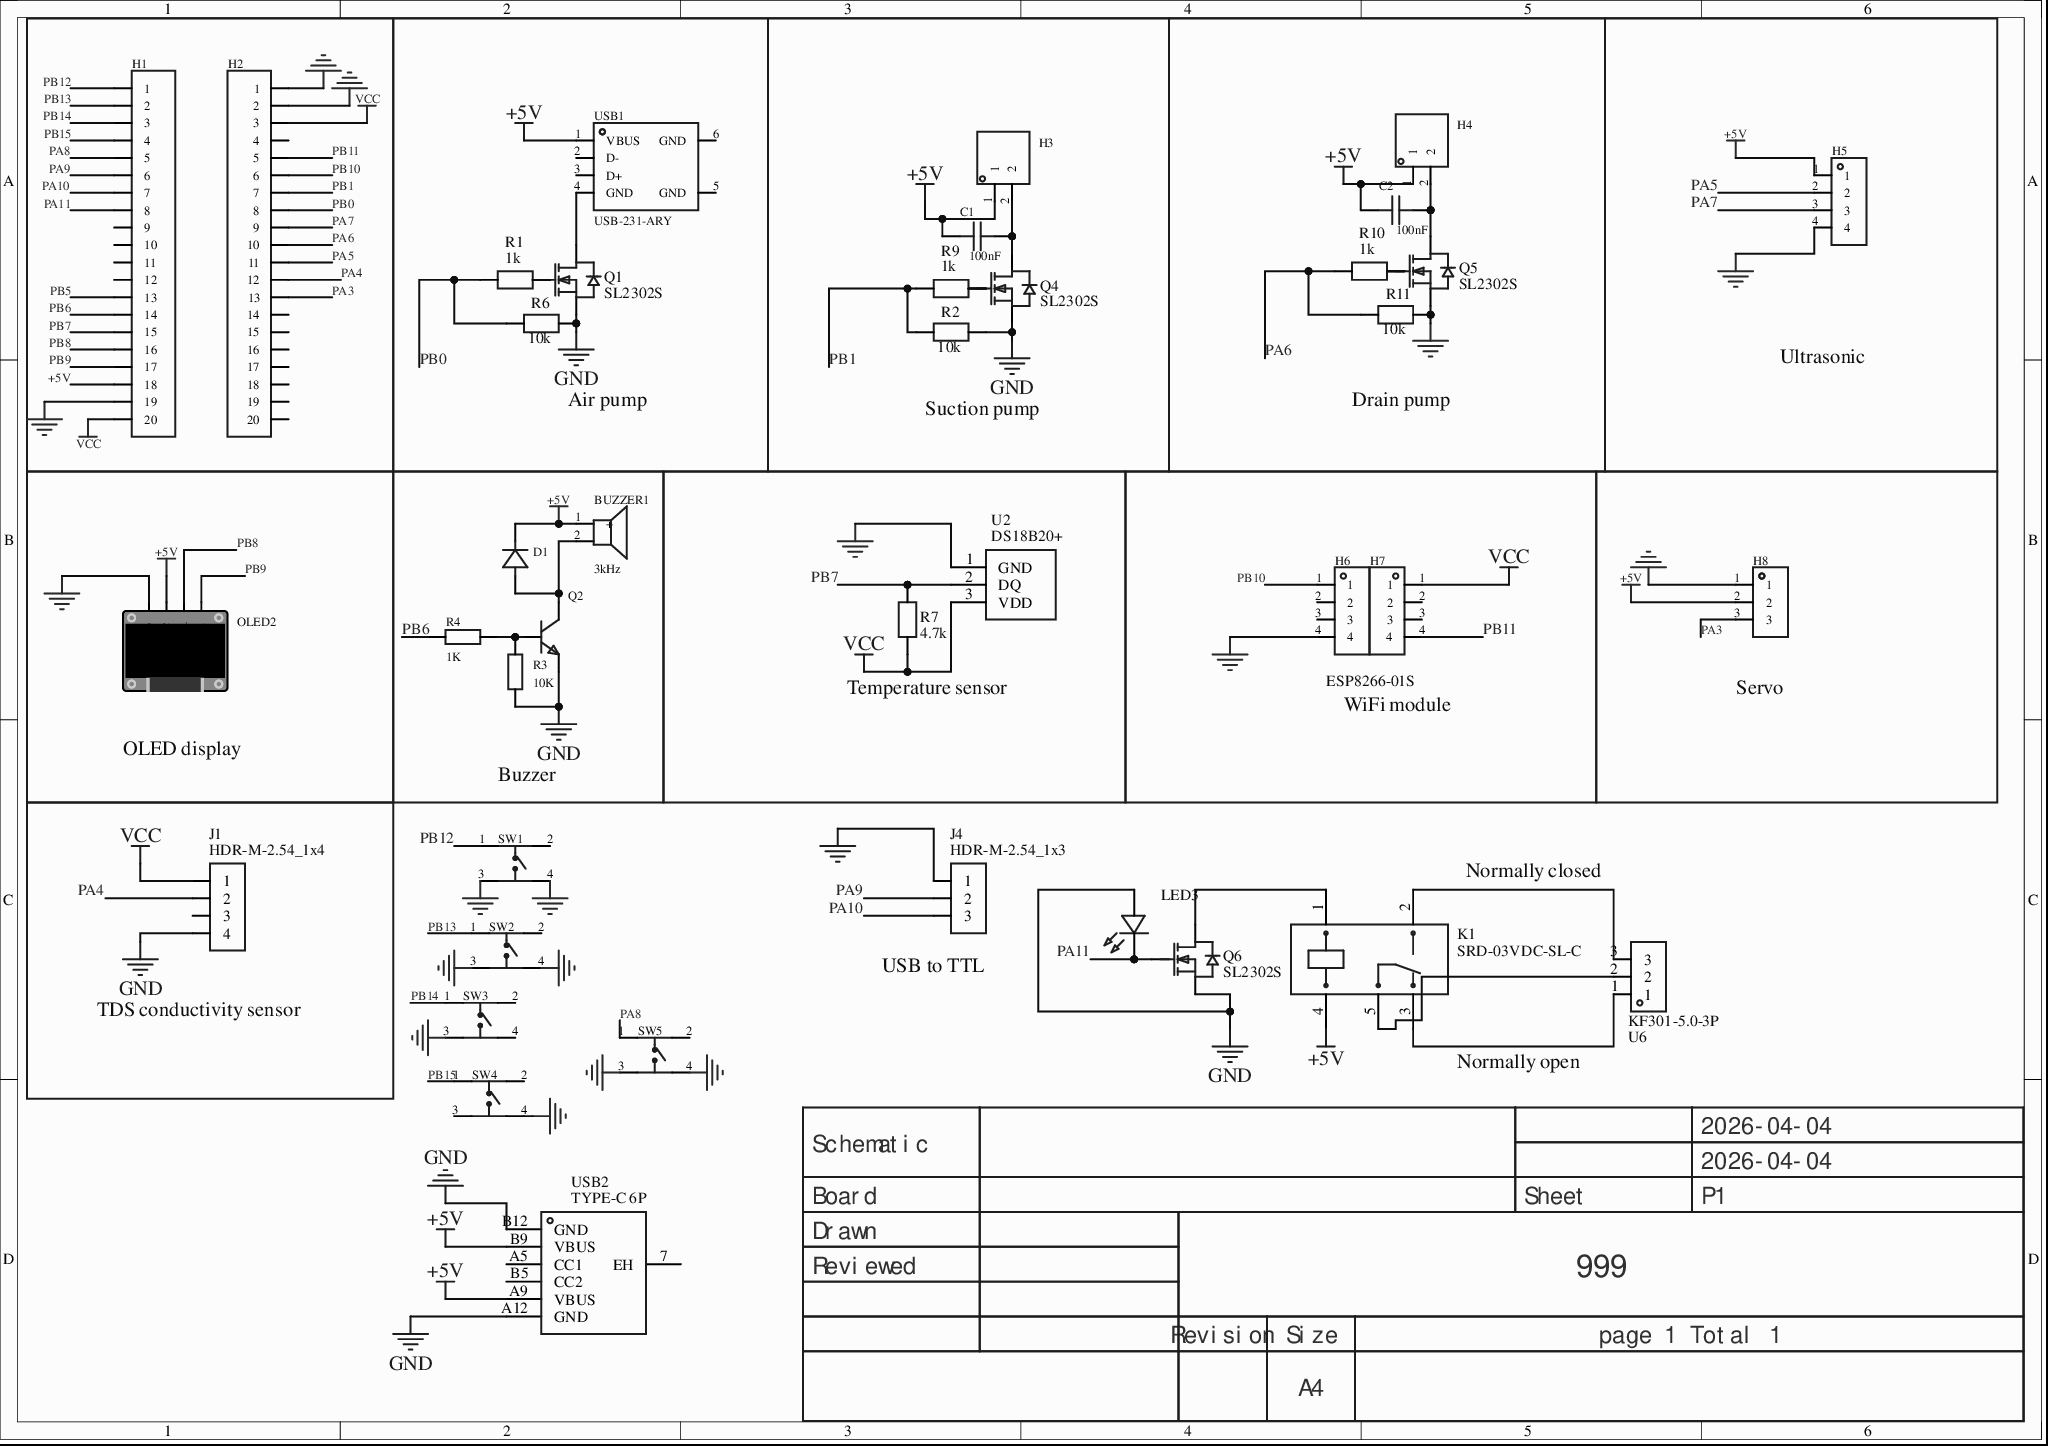
[diagram p0: MISC75353-3.schdoc]
# Altium project MISC75353-2.PrjPcb
1 sheet, 40 parts. Net scope: global (net labels, ports and power ports of the same name join across sheets).
Board file: MISC75353.pcbdoc

## Sheet MISC75353-3.schdoc
size 297 x 209 mm; Version: V1.0; @Project Name: MISC75353; @Update Date: 2026-04-04; @Create Date: 2026-04-04; @Board Name: MISC75353; @Create Time: 13:37:19; @Page Count: 1; @Page No: 1; @Schematic Name: MISC75353; @Update Time: 13:37:19; Size: A4

### Parts
BUZZER1  3kHz  [BUZ-TH_BD9.6-P5.00-D0.7-FD]
C1  100nF  [C0805]
C2  100nF  [C0805]
D1  (no value)  [DO_1N4007]
H1  (no value)  [HDR-TH_20P-P2.54-V-F]
H2  (no value)  [HDR-TH_20P-P2.54-V-F]
H3  (no value)  [HDR-TH_2P-P2.54-V-M-1]
H4  (no value)  [HDR-TH_2P-P2.54-V-M-1]
H5  (no value)  [HDR-TH_4P-P2.54-V-M]
H6  (no value)  [HDR-TH_4P-P2.54-V-M]
H7  (no value)  [HDR-TH_4P-P2.54-V-M]
H8  (no value)  [HDR-TH_3P-P2.54-V-M]
J1  HDR-M-2.54_1x4  [HDR-M-2.54_1X4]
J4  HDR-M-2.54_1x3  [HDR-M-2.54_1X3]
K1  SRD-03VDC-SL-C  [RELAY-TH_SRD-XXVDC-XL-C]
LED3  LED-TH-5mm_R  [LED-TH_BD5.0_RED]  (value not drawn)
OLED2  (no value)  [0.96OLED_4P]
Q1  SL2302S  [SOT-23_L2.9-W1.3-P1.90-LS2.4-BR]
Q2  (no value)  [S8050_TO_92]
Q4  SL2302S  [SOT-23_L2.9-W1.3-P1.90-LS2.4-BR]
Q5  SL2302S  [SOT-23_L2.9-W1.3-P1.90-LS2.4-BR]
Q6  SL2302S  [SOT-23_L2.9-W1.3-P1.90-LS2.4-BR]
R1  1k  [R0603]
R2  10k  [R0603]
R3  10K  [R0603]
R4  1K  [R0603]
R6  10k  [R0603]
R7  4.7k  [R0603]
R9  1k  [R0603]
R10  1k  [R0603]
R11  10k  [R0603]
SW1  J1L0503110  [SW-TH_4P-L6.0-W6.0-P4.50-LS6.3]  (value not drawn)
SW2  J1L0503110  [SW-TH_4P-L6.0-W6.0-P4.50-LS6.3]  (value not drawn)
SW3  J1L0503110  [SW-TH_4P-L6.0-W6.0-P4.50-LS6.3]  (value not drawn)
SW4  J1L0503110  [SW-TH_4P-L6.0-W6.0-P4.50-LS6.3]  (value not drawn)
SW5  J1L0503110  [SW-TH_4P-L6.0-W6.0-P4.50-LS6.3]  (value not drawn)
U2  DS18B20+  [TO-92-3_L4.9-W3.7-P1.27-L]
U6  KF301-5.0-3P  [CONN-TH_3P-P5.00_KF301-5.0-3P]
USB1  USB-231-ARY  [USB-A-TH_USB-231-ARY]
USB2  TYPE-C 6P  [TYPE-C-SMD_TYPE-C-6P_1]

### Blocks framed on the sheet
Air pump: Q1 R1 R6 USB1
Suction pump: C1 H3 Q4 R2 R9
Drain pump: C2 H4 Q5 R10 R11
Ultrasonic: H5
OLED display: OLED2
Buzzer: BUZZER1 D1 Q2 R3 R4
Temperature sensor: R7 U2
WiFi module: H6 H7
Servo: H8
TDS conductivity sensor: J1

### Nets
+5V: BUZZER1.1(+) C1.1 C2.1 D1.1(K) H1.18 H3.1 H4.1 H5.1 H8.2 K1.4 OLED2.2(VCC) USB1.1(VBUS) USB2.A9(VBUS) USB2.B9(VBUS)
GND: H1.19 H2.1 H2.2 H5.4 H6.4 H8.1 J1.4 J4.1 LED3.1 OLED2.1(GND) Q1.2(S) Q2.1(E) Q4.2(S) Q5.2(S) Q6.2(S) R2.2 R3.1 R6.2 R11.2 SW1.3 SW1.4 SW2.3 SW2.4 SW3.3 SW4.4 SW5.3 SW5.4 U2.1(GND) USB2.A12(GND) USB2.B12(GND)
VCC: H1.20 H2.3 H7.1 J1.1 R7.2 U2.3(VDD)
PA3: H2.13 H8.3
PA4: H2.12 J1.2
PA5: H2.11 H5.2
PA6: H2.10 R10.1 R11.1
PA7: H2.9 H5.3
PA8: H1.5 SW5.1
PA9: H1.6 J4.2
PA10: H1.7 J4.3
PA11: H1.8 LED3.2 Q6.1(G)
PB0: H2.8 R1.1 R6.1
PB1: H2.7 R2.1 R9.1
PB5: H1.13
PB6: H1.14 R4.2
PB7: H1.15 R7.1 U2.2(DQ)
PB8: H1.16 OLED2.3(SCL)
PB9: H1.17 OLED2.4(SDA)
PB10: H2.6 H6.1
PB11: H2.5 H7.4
PB12: H1.1 SW1.1
PB13: H1.2 SW2.1
PB14: H1.3 SW3.1
PB15: H1.4 SW4.1
NetBUZZER1_2: BUZZER1.2 D1.2(A) Q2.3(C)
NetC1_2: C1.2 H3.2 Q4.3(D)
NetC2_2: C2.2 H4.2 Q5.3(D)
NetK1_1: K1.1 Q6.3(D)
NetK1_2: K1.2 U6.3
NetK1_3: K1.3 U6.1
NetK1_5: K1.5 U6.2
NetQ1_1: Q1.1(G) R1.2
NetQ1_3: Q1.3(D) USB1.4(GND)
NetQ2_2: Q2.2(B) R3.2 R4.1
NetQ4_1: Q4.1(G) R9.2
NetQ5_1: Q5.1(G) R10.2

Not connected (* = marked no-connect by the designer): H1 9 10 11 12; H2 4 14 15 16 17 18 19 20; H6 2* 3*; H7 2* 3*; J1 3*; SW1 2*; SW2 2*; SW3 2* 4*; SW4 2* 3*; SW5 2*; USB1 2(D-)* 3(D+)* 5(GND)* 6(GND)*; USB2 7(EH)* A5(CC1)* B5(CC2)*

### Notes on the sheet
- ESP8266-01S
- Normally closed
- (near J4) USB to TTL
- Normally open
- 2026-04-04
- Schematic
- Board
- Sheet
- P1
- Drawn
- Reviewed
- 999
- Revision
- Size
- A4
- page 1 Total 1

### Library data of the parts
BUZZER1 = HNB09A05: Driver type: active (built-in driver circuit); construction type: electromagnetic; rated voltage: -; frequency: 3kHz; sound pressure (SPL): 85dB;; Manufacturer: 华能; 3D Model: 13273335caac486e928bafb4d9fdf12d0819f05c4eef4c71ace90d822a990e87; 3D Model Transform: 354.33,354.33,0,90,0,0,0,0,-177.165; Voltage - Supply: 3V~7V; AddInBom: yes; ModelName: BUZ-TH_D9.0-H5.5-P5.0; Symbol: HNB09A05; Device: HNB09A05; LCSC Part Name: HNB09A05; Supplier Part: C96493; Manufacturer Part: HNB09A05; Supplier Footprint: 插件,D=9mm; JLCPCB Part Class: Extended Part; Datasheet: https://example.com/datasheet/HNB09A05/97698.html; Supplier: LCSC; Driver Circuitry: Active (built-in driver circuit); Technology: Electromagnetic; Voltage Rating: -; Value: 3kHz; Current Consumption: -; Sound Pressure Level(SPL): 85dB; Diameter(φD): 9mm; Length: -; Width: -; Height: 5.7mm; Operating Temperature: -; ConvertToPcb: yes; FootprintName: BUZ-TH_BD9.6-P5.00-D0.7-FD
C1 C2 = CAP_0805: Symbol: Capacitance; ConvertToPcb: yes; ModelId: 1ba041120af144c991958decab20d2410819f05c4eef4c71ace90d822a990e87; ModelName: C0805_L2.0-W1.3-H1.3; ModelTransform: 78.74,51.181,0,0,0,0,0,0.0005,0; Device: CAP_0805; AddInBom: yes; Supplier Footprint: 0805; FootprintName: C0805; Value: 100nF
D1 = D_1N4007A: AddInBom: yes; ModelId: 6de1e9b71a0d4751b4e9df530304c1a30819f05c4eef4c71ace90d822a990e87; ModelName: DO-41_D2.4-L4.7-P8.70; ModelTransform: 373.9,94.4,232.29,0,0,0,0,0,-140; Symbol: D_1N4007; Device: D_1N4007A; Supplier Footprint: DO-41; ConvertToPcb: yes; FootprintName: DO_1N4007
H1 H2 = HDR-F_2.54_1x20P: 3D Model: db7015f7ad9d48b8a3b1188db02e34290819f05c4eef4c71ace90d822a990e87; 3D Model Transform: 1999.996,100,0,0,0,0,0,0,-118.11; ConvertToPcb: yes; ModelName: HDR-F-2.54_1x20; Symbol: HDR-F_2.54_1x20P; Device: HDR-F_2.54_1x20P; Supplier Part: C50984; Supplier Footprint: 插件; AddInBom: yes; FootprintName: HDR-TH_20P-P2.54-V-F
H3 H4 = HDR-M_2.54_1x2P: Symbol: 210S-1*2P L=11.6MMGold-plated black; ConvertToPcb: yes; ModelId: 79b2e9f2d70a4d68a1b7098f27c6d4c50819f05c4eef4c71ace90d822a990e87; ModelName: HDR-M-2.54_1x2; ModelTransform: 200,100,0,0,0,0,0,0,-118.11; Device: HDR-M_2.54_1x2P; AddInBom: yes; SupplierPart: C124375; Supplier Footprint: 插件; FootprintName: HDR-TH_2P-P2.54-V-M-1
H5-H7 = HDR-M_2.54_1x4P: Symbol: PZ254V-11-04P; ConvertToPcb: yes; ModelId: 112f4d05e8d64e99ab9a333894bea4f90819f05c4eef4c71ace90d822a990e87; ModelName: HDR-TH_4P-P2.54-M-LI-1X4P; ModelTransform: 399.999,104.7242,0,0,0,0,0,0,-118.11; Device: HDR-M_2.54_1x4P; AddInBom: yes; SupplierPart: C492403; Supplier Footprint: 插件; FootprintName: HDR-TH_4P-P2.54-V-M
H8 = HDR-M_2.54_1x3P: AddInBom: yes; ModelId: bb473b6d38ff42a99216a4fcdbdcc4cb0819f05c4eef4c71ace90d822a990e87; ModelName: HDR-TH_3P-P2.54-M-LI-1X3P; ModelTransform: 300.03877,100,0,0,0,0,0,0,-118.11; Symbol: HDR-M_2.54_1x3P; Device: HDR-M_2.54_1x3P; ConvertToPcb: yes; FootprintName: HDR-TH_3P-P2.54-V-M; SupplierPart: C2937625; Supplier Footprint: 插件
J1 = HDR-M-2.54_1x4: Add into BOM: yes; ModelId: cd502121c3eb48dbbf0ecbc8e7ad097f; Symbol: HDR-M-2.54_1x4; Device: HDR-M-2.54_1x4; Convert to PCB: yes; Supplier Part: C124378; Supplier: LCSC; Origin 3D Model Title: HDR-M-2.54_1X4; FootprintName: HDR-M-2.54_1X4; ModelName: HDR-M-2.54_1X4
J4 = HDR-M-2.54_1x3: Add into BOM: yes; ModelId: e45037aab22c4927a5ea885f2a5b96c9; Symbol: HDR-M-2.54_1x3; Device: HDR-M-2.54_1x3; Convert to PCB: yes; Supplier Part: C180248; Supplier: LCSC; Origin 3D Model Title: HDR-M-2.54_1x3; FootprintName: HDR-M-2.54_1X3; ModelName: HDR-M-2.54_1x3
K1 = SRD-03VDC-SL-C: Manufacturer: 松乐; Add into BOM: yes; Origin 3D Model Title: RELAY-TH_L19.2-W15.6-H15.8; ModelId: d0eda9b8bf8746d18ae810ab88dc78e7; Symbol: SRD-03VDC-SL-C; Device: SRD-03VDC-SL-C; Convert to PCB: yes; Supplier: LCSC; Manufacturer Part: SRD-03VDC-SL-C; Supplier Part: C24585; JLCPCB Part Class: Extended Part; FootprintName: RELAY-TH_SRD-XXVDC-XL-C; ModelName: RELAY-TH_L19.2-W15.6-H15.8
LED3 = LED-TH-5mm_R: Manufacturer: EVERLIGHT(台湾亿光); Manufacturer Part: 333-2SURD/S530-A3; Add into BOM: yes; ModelId: 0e3e1c3f5c0d4d279dc0d0ab1929e6bc; Symbol: LED-TH-5mm_R; Device: LED-TH-5mm_R; Convert to PCB: yes; Supplier Part: C87271; Supplier: LCSC; Origin 3D Model Title: LED-TH_BD5.0_Red; FootprintName: LED-TH_BD5.0_RED; ModelName: LED-TH_BD5.0_Red
OLED2 = 0.96OLED模块_4P: Symbol: 0.96OLED module_4P; ConvertToPcb: yes; ModelId: 79c000fdb68d45a296c2e9bedf4f90550819f05c4eef4c71ace90d822a990e87; ModelTransform: 1393.69792,1318.895,0,0,0,0,0,-560.079,-137.795; Device: 0.96OLED module_4P; AddInBom: yes; FootprintName: 0.96OLED_4P; Supplier Footprint: 插件; ModelName: 0.96OLED_4P
Q1 Q4-Q6 = SL2302S: Manufacturer: Slkor(萨科微); Add into BOM: yes; Origin 3D Model Title: SOT-23-3P_L2.9-W1.3-H1.0-LS2.4-P0.95; ModelId: c62791f0466c4ae2a892c056b845b0ca; Symbol: SL2302S; Device: SL2302S; Convert to PCB: yes; Supplier: LCSC; Supplier Part: C473811; Manufacturer Part: SL2302S; JLCPCB Part Class: Extended Part; FootprintName: SOT-23_L2.9-W1.3-P1.90-LS2.4-BR; ModelName: SOT-23-3P_L2.9-W1.3-H1.0-LS2.4-P0.95
Q2 = S8050_TO_NPN: ConvertToPcb: yes; ModelId: aafe8e06f2154e7c93506efd0d6632dd0819f05c4eef4c71ace90d822a990e87; ModelName: TO-92-3_L4.9-W3.7-P1.27-L; ModelTransform: 180.78,141.44,417.3,0,0,0,0,0,-200; Symbol: S8050_TO_NPN; Device: S8050_TO_NPN; AddInBom: yes; Supplier Footprint: TO-92; FootprintName: S8050_TO_92
R1 R9 R10 = 1k: Add into BOM: yes; ModelId: fc143cca1e79419f9cd78b61e9279f08; Symbol: 1k; Device: 1k; Convert to PCB: yes; Origin 3D Model Title: R0603; FootprintName: R0603; ModelName: R0603
R2 R6 R7 R11 = 10k: Add into BOM: yes; ModelId: fc143cca1e79419f9cd78b61e9279f08; Symbol: 10k; Device: 10k; Convert to PCB: yes; Origin 3D Model Title: R0603; FootprintName: R0603; ModelName: R0603
R3 R4 = Res_0603: Symbol: Resistor; ConvertToPcb: yes; ModelId: fc143cca1e79419f9cd78b61e9279f080819f05c4eef4c71ace90d822a990e87; ModelTransform: 31.8897,63.7794,0,90,0,0,0,0,0; Device: Res_0603; AddInBom: yes; Supplier Footprint: 0603; FootprintName: R0603; ModelName: R0603
  R3: Value: 10K
  R4: Value: 1K
SW1 = J1L0503110: 电路结构:单刀单掷;按钮形状:圆形按钮;作用力:2.6N;安装方式:直插;开关长度:6mm;开关宽度:6mm;开关高度:5mm;带支架:-;触点电流:50mA;额定电压:12V;带灯:无;工作寿命:10万次;; Manufacturer: SAMZO(三佐); 3D Model: f12d4fb4f8314a3f92db4aebb329b4320819f05c4eef4c71ace90d822a990e87; 3D Model Transform: 306.99781,236.22,0,0,0,0,0,0,-137.795; Circuit: SPST; Actuator Style: Round button; Operating Force: 2.6N; Switch Height: 5mm; Contact Current: 50mA; Voltage Rating: 12V; Actuator/Cap Color: Black; With Lamp: None; Life: 10万 cycles; AddInBom: yes; Description: Circuit structure: SPST; button shape: round button; actuating force: 2.6N; mounting: through-hole; switch length: 6mm; switch width: 6mm; switch height: 5mm; with bracket: -; contact current: 50mA; rated voltage: 12V; with lamp: none; life: 10万 cycles;; Symbol: J1L0503110; Device: J1L0503110; LCSC Part Name: 6*6*5 四脚插件 铜盖 260gf; Supplier Part: C29780808; Manufacturer Part: J1L0503110; Supplier Footprint: 插件-4P,6x6mm; JLCPCB Part Class: Extended Part; Datasheet: https://example.com/datasheet/J1L0503110/31512971.html; Supplier: LCSC; Mounting Type: Through-hole; Length: 6mm; Width: 6mm; with Bracket: -; IP Rating: -; Termination Style: -; Operating Temperature: -25℃~+85℃; ConvertToPcb: yes; FootprintName: SW-TH_4P-L6.0-W6.0-P4.50-LS6.3; ModelName: SW-TH_4P-L6.0-W6.0-P4.50-LS6.3
SW2-SW5 = J1L0503110: Circuit structure: SPST; button shape: round button; actuating force: 2.6N; mounting: through-hole; switch length: 6mm; switch width: 6mm; switch height: 5mm; with bracket: -; contact current: 50mA; rated voltage: 12V; with lamp: none; life: 10万 cycles;; Manufacturer: SAMZO(三佐); 3D Model: f12d4fb4f8314a3f92db4aebb329b4320819f05c4eef4c71ace90d822a990e87; 3D Model Transform: 306.99781,236.22,0,0,0,0,0,0,-137.795; Actuator/Cap Color: Black; AddInBom: yes; Symbol: J1L0503110; Device: J1L0503110; LCSC Part Name: 6*6*5 四脚插件 铜盖 260gf; Supplier Part: C29780808; Manufacturer Part: J1L0503110; Supplier Footprint: 插件-4P,6x6mm; JLCPCB Part Class: Extended Part; Datasheet: https://example.com/datasheet/J1L0503110/31512971.html; Supplier: LCSC; Circuit: SPST; Actuator Style: Round button; Operating Force: 2.6N; Mounting Type: Through-hole; Length: 6mm; Width: 6mm; Switch Height: 5mm; with Bracket: -; Contact Current: 50mA; Voltage Rating: 12V; With Lamp: None; IP Rating: -; Termination Style: -; Life: 10万 cycles; Operating Temperature: -25℃~+85℃; ConvertToPcb: yes; FootprintName: SW-TH_4P-L6.0-W6.0-P4.50-LS6.3; ModelName: SW-TH_4P-L6.0-W6.0-P4.50-LS6.3
U2 = DS18B20+: Manufacturer: ADI(亚德诺)/MAXIM(美信); Add into BOM: yes; ModelId: aafe8e06f2154e7c93506efd0d6632dd; Symbol: DS18B20+; Device: DS18B20+; Convert to PCB: yes; Supplier: LCSC; Manufacturer Part: DS18B20+; Supplier Part: C9753; JLCPCB Part Class: Extended Part; Origin 3D Model Title: TO-92-3_L4.9-W3.7-P1.27-L; FootprintName: TO-92-3_L4.9-W3.7-P1.27-L; ModelName: TO-92-3_L4.9-W3.7-P1.27-L
U6 = KF301-5.0-3P: Manufacturer: KEFA(科发); Add into BOM: yes; ModelId: 7090fd1e13c24e5e88660dd73c452457; Symbol: KF301-5.0-3P; Device: KF301-5.0-3P; Convert to PCB: yes; Supplier: LCSC; Supplier Part: C474882; Manufacturer Part: KF301-5.0-3P; JLCPCB Part Class: Extended Part; Origin 3D Model Title: CONN-TH_3P-P5.00_KF301-5.0-3P; FootprintName: CONN-TH_3P-P5.00_KF301-5.0-3P; ModelName: CONN-TH_3P-P5.00_KF301-5.0-3P
USB1 = USB-231-ARY: Connector type: Type-A; protocol standard: USB 2.0; gender: female; mounting: right angle; contact count: 4P; port count: 1; rated current - power: 1.5A; operating temperature: -20℃~+70℃;; Manufacturer: XUNPU(讯普); AddInBom: yes; ModelId: 2c22904cfa634797a8992a7288a8f2530819f05c4eef4c71ace90d822a990e87; ModelTransform: 610.18209,551.18,0,0,0,0,0,-183.071,-137.795; Protocol Standard: USB 2.0; Number of Ports: 1; Voltage Rating: 30V; Detection color: White; Symbol: USB-231-ARY; Device: USB-231-ARY; LCSC Part Name: Type-A 母 弯插; SupplierPart: C720525; ManufacturerPart: USB-231-ARY; Supplier Footprint: 弯插; JLCPCB Part Class: Extended Part; Datasheet: https://example.com/datasheet/USB-231-ARY/763532.html; Supplier: LCSC; ConvertToPcb: yes; FootprintName: USB-A-TH_USB-231-ARY; ModelName: USB-A-TH_USB-231-ARY; Connector Type: Type-A; Gender: Female; Mounting Type: Right angle; Number of Contacts: 4P; Current Rating-Power: 1.5A; Length: 14.2mm; Operating Temperature: -20℃~+70℃
USB2 = TYPE-C 6P: Manufacturer: SHOU HAN(首韩); Add into BOM: yes; Origin 3D Model Title: TYPE-C-SMD_6P-L8.9-W6.8-H3.2-P1.00; ModelId: 3770c5585474407db939b2377e27177a; Symbol: TYPE-C 6P; Device: TYPE-C 6P; Convert to PCB: yes; Supplier: LCSC; Supplier Part: C456012; Manufacturer Part: TYPE-C 6P; JLCPCB Part Class: Extended Part; FootprintName: TYPE-C-SMD_TYPE-C-6P_1; ModelName: TYPE-C-SMD_6P-L8.9-W6.8-H3.2-P1.00